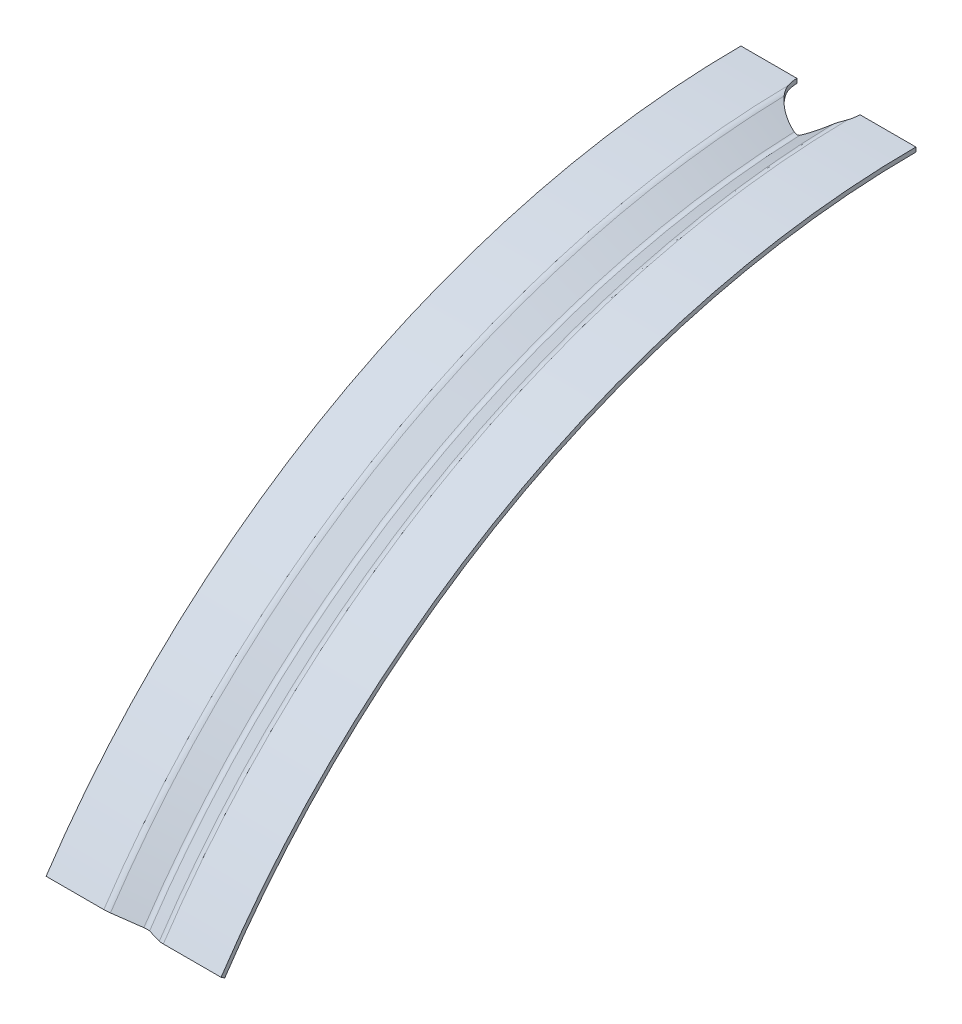
from build123d import *

# Parameters (mm, degrees)
SKETCH3_R          = 57.15
CUT_EXTRUDE1_DEPTH = 50


with BuildPart() as part:
    # Sweep1: sweep along a path in Sketch2
    with BuildLine(Plane(origin=(0, 0, 0), x_dir=(0, 0, -1), z_dir=(1, 0, 0))) as sweep1_path:
        ThreePointArc((0, 20.7), (-715, -158.48445696), (-1260.994295686, -653.683708467))
    # Sketch1 → Sweep1 (sweep)
    with BuildSketch(Plane.XY):
        with BuildLine():
            Line((-158.75, 20.7), (-53.975, 20.7))
            ThreePointArc((-53.975, 20.7), (-48.941078797, 19.961460685), (-44.331437049, 17.808089852))
            Line((-44.331437049, 17.808089852), (-5.241365883, -7.953220019))
            ThreePointArc((-5.241365883, -7.953220019), (0, -9.525), (5.241365883, -7.953220019))
            Line((5.241365883, -7.953220019), (44.331437049, 17.808089852))
            ThreePointArc((44.331437049, 17.808089852), (48.941078797, 19.961460685), (53.975, 20.7))
            Line((53.975, 20.7), (158.75, 20.7))
            Line((158.75, 20.7), (158.75, 12.7))
            Line((158.75, 12.7), (53.975, 12.7))
            ThreePointArc((53.975, 12.7), (51.23901715, 12.298597034), (48.733634117, 11.128220019))
            Line((48.733634117, 11.128220019), (9.643562951, -14.633089852))
            ThreePointArc((9.643562951, -14.633089852), (0, -17.525), (-9.643562951, -14.633089852))
            Line((-9.643562951, -14.633089852), (-48.733634117, 11.128220019))
            ThreePointArc((-48.733634117, 11.128220019), (-51.23901715, 12.298597034), (-53.975, 12.7))
            Line((-53.975, 12.7), (-158.75, 12.7))
            Line((-158.75, 12.7), (-158.75, 20.7))
        make_face()
    sweep(path=sweep1_path.line)

    # Sketch3 → Cut-Extrude1 (cut, symmetric)
    with BuildSketch(Plane(origin=(0, 0, 0), x_dir=(1, 0, 0), z_dir=(0, 1, 0))):
        Circle(SKETCH3_R)
    extrude(amount=CUT_EXTRUDE1_DEPTH, both=True, mode=Mode.SUBTRACT)


solid = part.part
